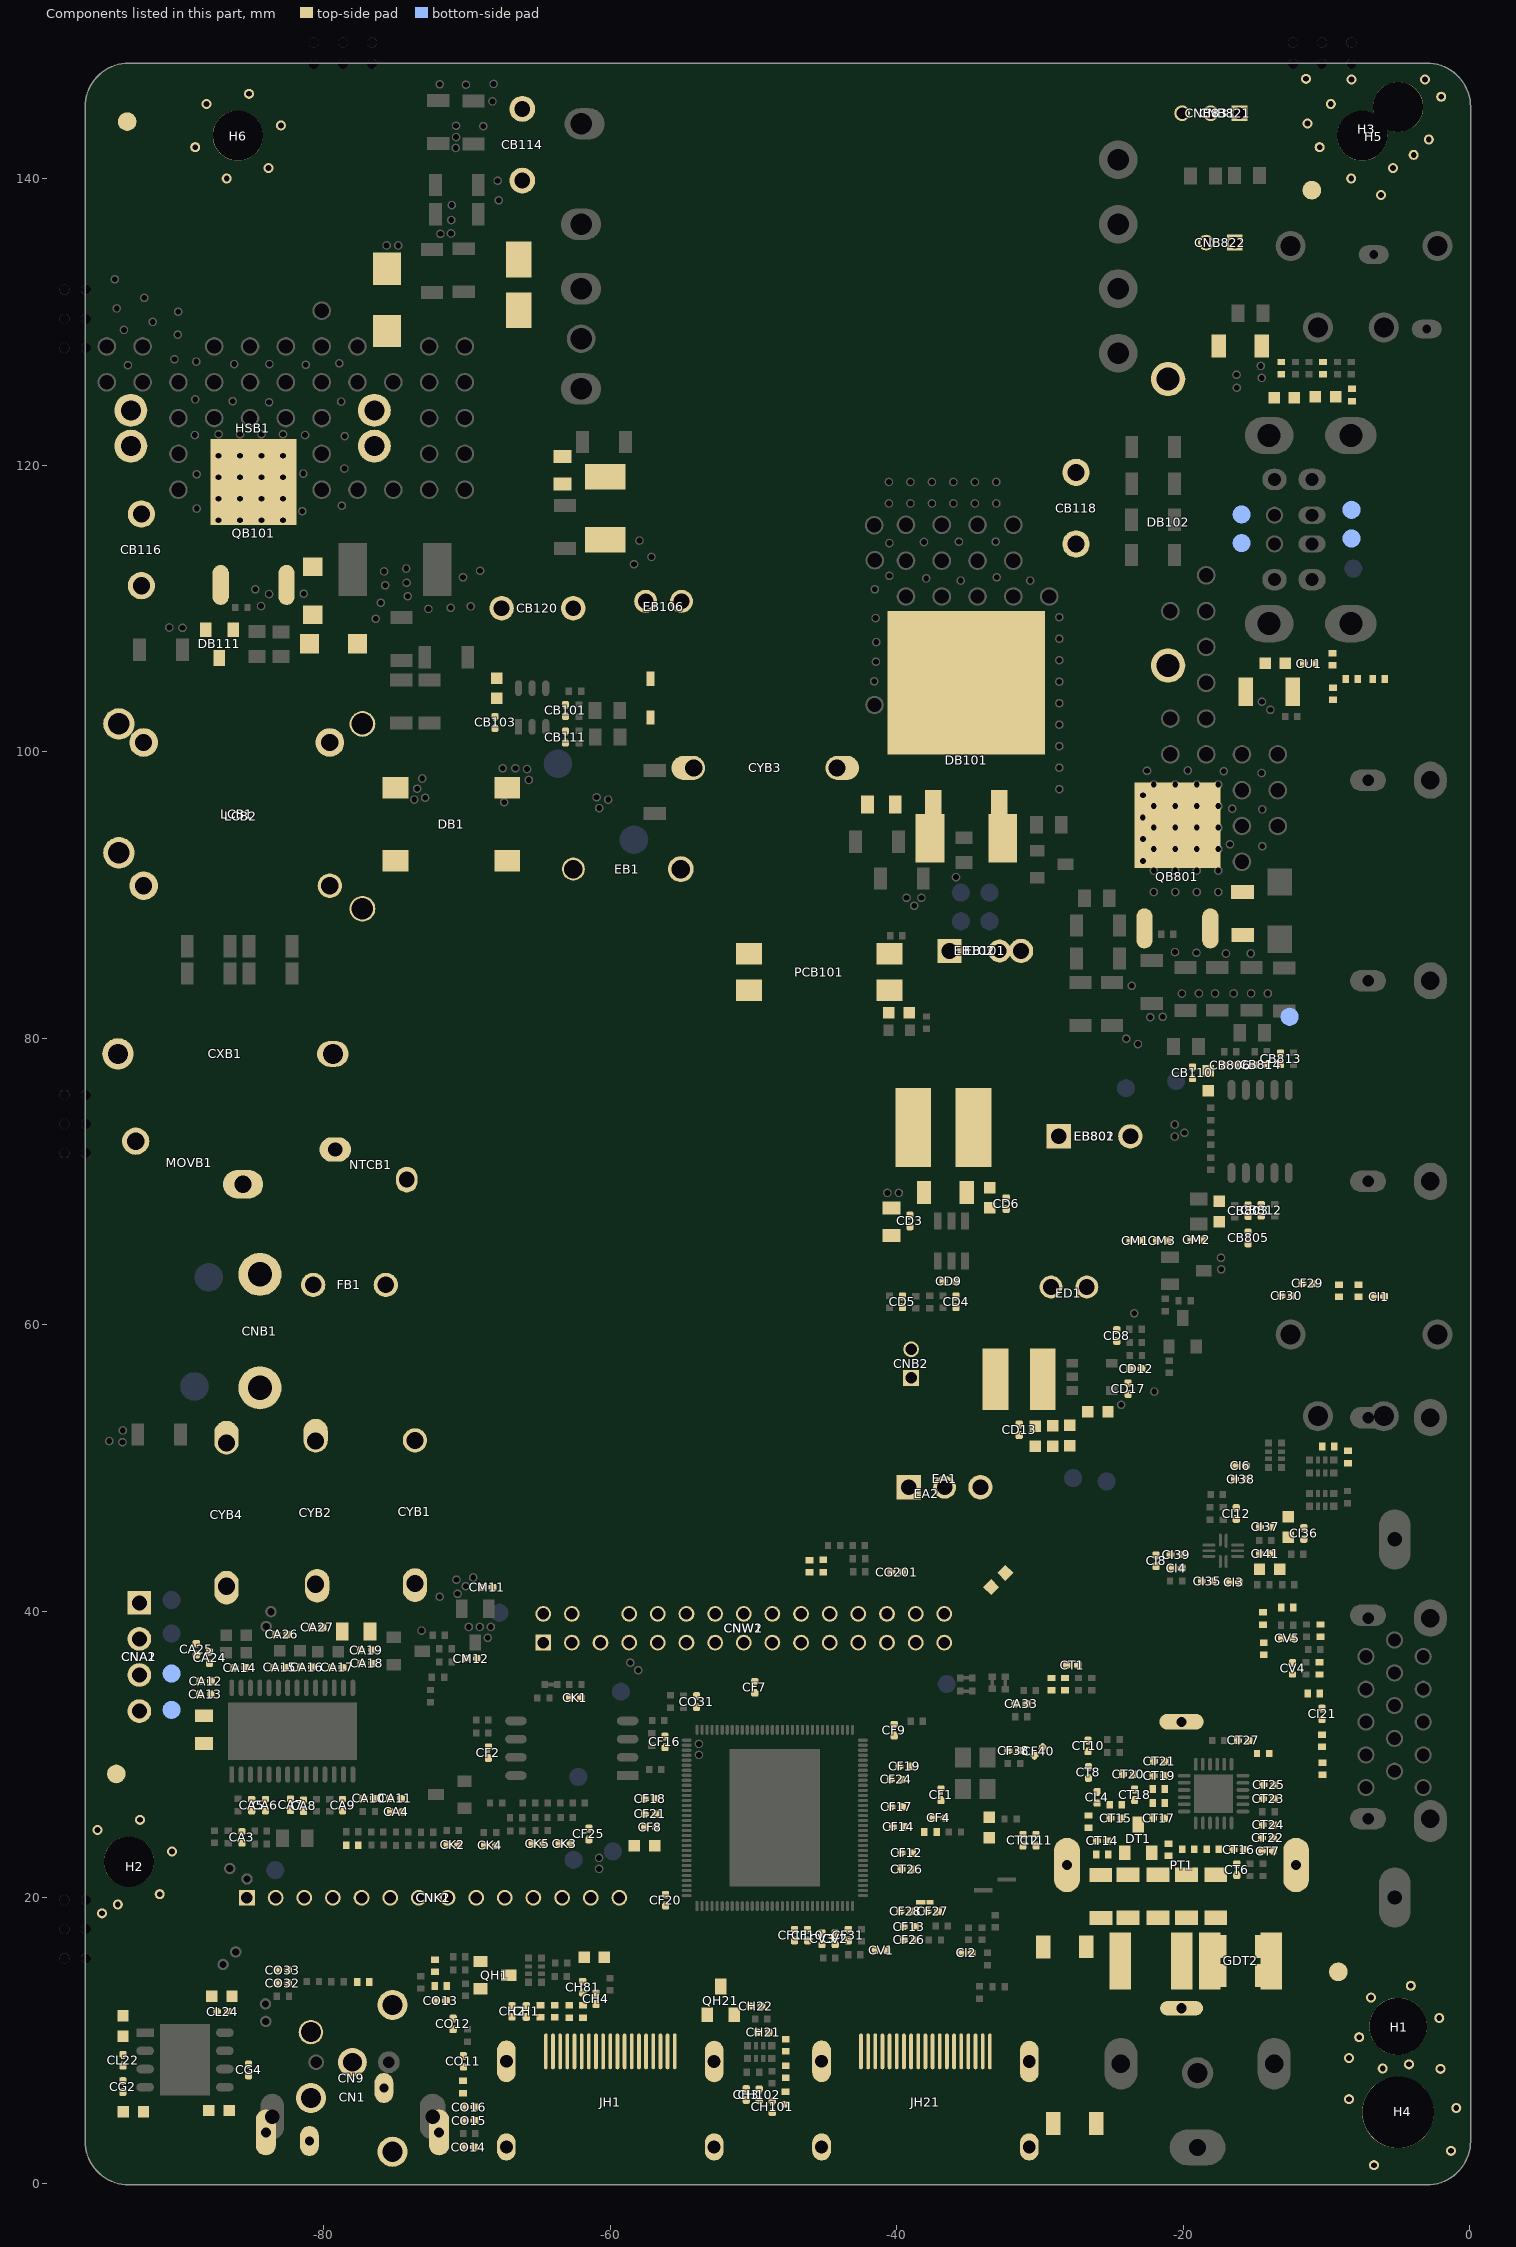
[diagram p0: the components of this part, seen from the top]
# Altium PCB MISC86372.PcbDoc (part 2 of 16)
Units mm, origin at the board's own origin, x right, y up, seen from the top; angles counter-clockwise.
Board outline 96.73 x 148.13 mm, 2 copper layers (TopLayer, BottomLayer), stack 1.571 mm thick; 578 components, 318 nets, 2702 pads, 836 vias.

## Components (designator, comment, footprint, x,y, rotation, side; value= is the part's Value field where it differs from the comment) (continued)
BB101 "Ferrite bead,BEAD,50ohm,3.0×4.0mm,9A,SMD,TP,BPH403025W4-470T,TAI-TECH" L(4*3*2.55)-S -66.396,132.585 r90 top
CA1 "10uF-0805-X5R-±20%-16V" C0805 -88.367,31.725 r90 top
CA2 "NC/10uF-0805-X5R-±20%-16V" C0805 -77.749,38.583 r180 top
CA3 "3300pF-0402-X7R-±10%-50V" C0402 -85.714,24.197 r90 top
CA4 "3300pF-0402-X7R-±10%-50V" C0402 -74.939,25.984 r180 top
CA5 "0.22uF-0402-X5R-±10%-16V" C0402 -85.033,26.448 r90 top
CA6 "0.22uF-0402-X5R-±10%-16V" C0402 -84.075,26.448 r90 top
CA7 "1uF-0402-X5R-±20%-16V" C0402 -82.324,26.468 r90 top
CA8 "1uF-0402-X5R-±20%-16V" C0402 -81.416,26.406 r90 top
CA9 "1uF-0402-X5R-±20%-16V" C0402 -78.689,26.448 r90 top
CA10 "0.22uF-0402-X5R-±10%-16V" C0402 -76.864,26.92 r180 top
CA11 "0.22uF-0402-X5R-±10%-16V" C0402 -74.994,26.921 r180 top
CA12 "NC/0.1uF-0402-X5R-±20%-16V" C0402 -88.243,35.105 r0 top
CA13 "1000pF-0402-X7R-±10%-50V" C0402 -88.268,34.188 r0 top
CA14 "0.22uF-0402-X5R-±10%-16V" C0402 -85.852,36.043 r0 top
CA15 "0.22uF-0402-X5R-±10%-16V" C0402 -83.077,36.069 r180 top
CA16 "0.22uF-0402-X5R-±10%-16V" C0402 -81.208,36.086 r0 top
CA17 "0.22uF-0402-X5R-±10%-16V" C0402 -79.063,36.068 r180 top
CA18 "NC/0.1uF-0402-X5R-±20%-16V" C0402 -76.995,36.347 r180 top
CA19 "1000pF-0402-X7R-±10%-50V" C0402 -77.025,37.272 r180 top
CA24 "2200pF-0402-X7R-±10%-50V" C0402 -87.979,36.751 r270 top
CA25 "2200pF-0402-X7R-±10%-50V" C0402 -88.9,37.338 r270 top
CA26 "2200pF-0402-X7R-±10%-50V" C0402 -82.927,38.372 r180 top
CA27 "2200pF-0402-X7R-±10%-50V" C0402 -80.463,38.869 r0 top
CA31 "10uF-0603-X5R-±20%-6.3V" C0603 -12.954,124.714 r180 top
CA32 "10uF-0603-X5R-±20%-6.3V" C0603 -10.062,124.765 r180 top
CA33 "Ceramic capacitor,CAP MC,6.3V,0.47uF,±10%,X5R,0402,SMD,TP" C0402 -31.323,33.528 r0 top
CAUTION "CAUTION" CAUTION -87.935,84.353 r90 bottom
CB101 "Ceramic capacitor,CAP MC,50V,100pF,±5%,NPO,0402,SMD,TP" C0402 -63.129,102.87 r270 top
CB102 "0.1uF-0603-X7R-±10%-50V" C0603 -67.92,104.419 r270 top
CB103 "Ceramic capacitor,CAP MC,50V,1000pF,±10%,X7R,0402,SMD,TP" C0402 -68.047,102.032 r90 top
CB109 "Ceramic capacitor,CAP MC,25V,0.22uF,±10%,X7R,0603,SMD,TP" C0603 -18.263,77.013 r270 top
CB110 "Ceramic capacitor,CAP MC,50V,100pF,±5%,NPO,0402,SMD,TP" C0402 -19.355,77.572 r270 top
CB111 "NC/Ceramic capacitor,CAP MC,50V,100pF,±5%,NPO,0402,SMD,TP" C0402 -63.129,101.016 r270 top
CB114 "Film capacitor,CAP PE,400V,4700pF,±5%,P,5.0mm,PC,DIP,TP,Fara" CAP8*2.5-V-5 -66.142,142.365 r90 top
CB116 "Ceramic capacitor,CAP CD,2KV,47pF,±5%,SL,IK,5.0mm,DIP,TP,Walsin" CAP7.5*5-V-5-1 -92.735,114.082 r270 top
CB117 "1000pF-0805-NPO-±10%-200V" C0805 -41.072,96.317 r180 top
CB118 "Ceramic capacitor,CAP CD,2KV,100pF,±5%,SL,IK,5.0mm,DIP,TP,Walsin" CAP8.5*5-V-5 -27.483,116.992 r270 top
CB119 "NC/1000pF-0805-NPO-±10%-200V" C0805 -63.348,119.634 r90 top
CB120 "NC/Ceramic capacitor,CAP CD,1KV,4700pF,±20%,Y5U,K,5.0mm,DIP,TP,Walsin" CAP10*4.5-V-5 -65.086,110.007 r0 top
CB129 "NC/Ceramic capacitor,CAP MC,1KV,1000pF,±5%,NPO,1206,SMD,TP" C1206 -15.85,88.697 r270 top
CB139 "NC/Ceramic capacitor,CAP MC,50V,0.022uF,±10%,X7R,0402,SMD,TP" C0603 -39.848,81.761 r180 top
CB801 "Ceramic capacitor,CAP MC,25V,1uF,±10%,X7R,0603,SMD,TP" C0603 -17.501,67.894 r270 top
CB803 "Ceramic capacitor,CAP MC,25V,0.1uF,±10%,X7R,0402,SMD,TP" C0402 -15.469,67.945 r270 top
CB805 "Ceramic capacitor,CAP MC,50V,0.01uF,±10%,X7R,0402,SMD,TP" C0402 -15.469,66.044 r270 top
CB806 "Ceramic capacitor,CAP MC,50V,1000pF,±10%,X7R,0402,SMD,TP" C0402 -16.713,78.105 r0 top
CB808 "NC/Ceramic capacitor,CAP MC,1KV,1000pF,±5%,NPO,1206,SMD,TP" C1206 -16.027,128.321 r180 top
CB812 "Ceramic capacitor,CAP MC,50V,220pF,±5%,NPO,0402,SMD,TP" C0402 -14.554,67.97 r90 top
CB813 "Ceramic capacitor,CAP MC,50V,100pF,±5%,NPO,0402,SMD,TP" C0402 -13.208,78.562 r270 top
CB814 "NC/100pF-0402-NPO-±5%-50V" C0402 -14.58,78.13 r180 top
CD1 "NC/10uF-1206-X5R-±10%-16V" C1206 -36.603,69.212 r180 top
CD2 "10uF-0805-X5R-±20%-16V" C0805 -40.361,67.168 r270 top
CD3 "NC/0.1uF-0402-X5R-±20%-16V" C0402 -39.079,67.231 r90 top
CD4 "0.1uF-0402-X5R-±20%-16V" C0402 -35.859,61.595 r90 top
CD5 "NC/56pF-0402-NPO-±5%-50V" C0402 -39.603,61.589 r270 top
CD6 "NC/0.1uF-0402-X5R-±20%-16V" C0402 -32.36,68.445 r90 top
CD7 "10uF-0603-X5R-±20%-6.3V" C0603 -33.503,68.845 r90 top
CD8 "0.1uF-0402-X5R-±20%-16V" C0402 -24.638,59.233 r90 top
CD9 "NC/0.1uF-0402-X5R-±20%-16V" C0402 -36.366,63.017 r0 top
CD10 "NC/10uF-0603-X5R-±20%-6.3V" C0603 -27.911,52.248 r270 top
CD12 "NC/NC/3300pF-0402-X7R-±10%-50V" C0402 -23.298,56.911 r0 top
CD13 "NC/0.1uF-0402-X5R-±20%-16V" C0402 -31.453,52.654 r270 top
CD14 "10uF-0603-X5R-±20%-6.3V" C0603 -29.115,52.222 r270 top
CD15 "10uF-0603-X5R-±20%-6.3V" C0603 -30.341,52.206 r270 top
CD16 "10uF-0603-X5R-±20%-6.3V" C0603 -25.96,53.904 r0 top
CD17 "NC/0.1uF-0402-X5R-±20%-16V" C0402 -23.849,55.525 r270 top
CD101 "NC/NC?" DIODE-S0402 -46.096,43.12 r90 top
CD102 "NC/NC?" DIODE-S0402 -45.131,43.145 r90 top
CF1 "Ceramic capacitor,CAP MC,50V,18pF,±5%,NPO,0402,SMD,TP" C0402 -36.906,27.178 r270 top
CF2 "0.1uF-0402-X5R-±20%-16V" C0402 -68.504,30.115 r270 top
CF3 "10uF-0603-X5R-±20%-6.3V" C0603 -57.615,23.628 r0 top
CF4 "Ceramic capacitor,CAP MC,50V,18pF,±5%,NPO,0402,SMD,TP" C0402 -37.058,25.552 r180 top
CF5 "10uF-0603-X5R-±20%-6.3V" C0603 -61.112,15.824 r180 top
CF7 "0.1uF-0402-X5R-±20%-16V" C0402 -49.911,34.671 r270 top
CF8 "0.1uF-0402-X5R-±20%-16V" C0402 -57.202,24.914 r0 top
CF9 "0.1uF-0402-X5R-±20%-16V" C0402 -40.174,31.689 r270 top
CF10 "0.1uF-0402-X5R-±20%-16V" C0402 -46.226,17.375 r90 top
CF11 "0.1uF-0402-X5R-±20%-16V" C0402 -47.14,17.375 r270 top
CF12 "0.1uF-0402-X5R-±20%-16V" C0402 -39.294,23.114 r180 top
CF13 "0.1uF-0402-X5R-±20%-16V" C0402 -39.115,17.975 r180 top
CF14 "0.1uF-0402-X5R-±20%-16V" C0402 -39.875,24.942 r180 top
CF15 "10uF-0603-X5R-±20%-6.3V" C0603 -32.918,42.164 r225 top
CF16 "0.1uF-0402-X5R-±20%-16V" C0402 -56.185,30.861 r270 top
CF17 "0.1uF-0402-X5R-±20%-16V" C0402 -40.005,26.34 r180 top
CF18 "0.1uF-0402-X5R-±20%-16V" C0402 -57.209,26.898 r180 top
CF19 "0.1uF-0402-X5R-±20%-16V" C0402 -39.446,29.159 r0 top
CF20 "0.1uF-0402-X5R-±20%-16V" C0402 -56.138,19.813 r90 top
CF21 "Ceramic capacitor,CAP MC,6.3V,0.47uF,±10%,X5R,0402,SMD,TP" C0402 -57.201,25.832 r180 top
CF24 "Ceramic capacitor,CAP MC,6.3V,2.2uF,±20%,X5R,0402,SMD,TP" C0402 -40.03,28.245 r0 top
CF25 "Ceramic capacitor,CAP MC,6.3V,0.47uF,±10%,X5R,0402,SMD,TP" C0402 -61.493,24.435 r90 top
CF26 "0.047uF-0402-X7R-±10%-16V" C0402 -39.116,17.043 r0 top
CF27 "NC/0.1uF-0402-X5R-±20%-16V" C0402 -37.484,19.043 r180 top
CF28 "1uF-0402-X5R-±20%-6.3V" C0402 -39.359,19.039 r0 top
CF29 "NC/1000pF-0402-X7R-±10%-50V" C0402 -11.303,62.865 r180 top
CF30 "NC/1000pF-0402-X7R-±10%-50V" C0402 -12.77,62.001 r0 top
CF31 "0.047uF-0402-X7R-±10%-16V" C0402 -43.383,17.374 r270 top
CF38 "NC/30pF-0402-NPO-±5%-50V" C0402 -31.833,30.251 r0 top
CF40 "Ceramic capacitor,CAP MC,50V,0.01uF,±10%,X7R,0402,SMD,TP" C0402 -30.099,30.201 r225 top
CG1 "10uF-0603-X5R-±20%-6.3V" C0603 -93.294,5.055 r180 top
CG2 "NC/Ceramic capacitor,CAP MC,6.3V,2.2uF,±20%,X5R,0402,SMD,TP" C0402 -94.027,6.802 r270 top
CG3 "NC/10uF-0603-X5R-±20%-6.3V" C0603 -87.323,5.13 r0 top
CG4 "1uF-0402-X5R-±20%-6.3V" C0402 -85.25,7.959 r270 top
CG201 "NC/0.1uF-0402-X5R-±20%-16V" C0402 -40.005,42.723 r0 top
CH1 "NC/0.1uF-0402-X5R-±20%-16V" C0402 -65.862,12.043 r90 top
CH2 "NC/0.1uF-0402-X5R-±20%-16V" C0402 -66.861,12.049 r90 top
CH3 "NC/Ceramic capacitor,CAP MC,50V,22pF,±5%,NPO,0402,SMD,TP" C0402 -50.506,6.244 r270 top
CH4 "NC/Ceramic capacitor,CAP MC,50V,22pF,±5%,NPO,0402,SMD,TP" C0402 -61.006,12.929 r270 top
CH21 "NC/0.1uF-0402-X5R-±20%-16V" C0402 -49.313,10.59 r0 top
CH22 "NC/0.1uF-0402-X5R-±20%-16V" C0402 -49.828,12.421 r180 top
CH81 "Ceramic capacitor,CAP MC,6.3V,0.47uF,±10%,X5R,0402,SMD,TP" C0402 -61.925,13.745 r90 top
CH101 "NC/10pF-0402-NPO-±5%-50V" C0402 -48.692,5.385 r270 top
CH102 "NC/10pF-0402-NPO-±5%-50V" C0402 -49.604,6.223 r90 top
CI1 "NC/10pF-0402-NPO-±5%-50V" C0402 -6.35,61.951 r180 top
CI2 "0.047uF-0402-X7R-±10%-16V" C0402 -35.154,16.129 r180 top
CI3 "NC/0.1uF-0402-X5R-±20%-16V" C0402 -16.472,41.993 r0 top
CI4 "NC/0.1uF-0402-X5R-±20%-16V" C0402 -20.496,42.996 r0 top
CI6 "0.1uF-0402-X5R-±20%-16V" C0402 -16.007,50.126 r0 top
CI8 "0.1uF-0402-X5R-±20%-16V" C0402 -21.895,43.51 r90 top
CI9 "NC/NC/10uF-0603-X5R-±20%-6.3V" C0603 -12.675,45.872 r270 top
CI12 "NC/Ceramic capacitor,CAP MC,6.3V,0.47uF,±10%,X5R,0402,SMD,TP" C0402 -16.298,46.805 r90 top
CI21 "NC/NC/10pF-0402-NPO-±5%-50V" C0402 -10.312,32.817 r270 top
CI35 "NC/1000pF-0402-X7R-±10%-50V" C0402 -18.335,42.088 r0 top
CI36 "NC/0.1uF-0402-X5R-±20%-16V" C0402 -11.582,45.415 r270 top
CI37 "NC/Ceramic capacitor,CAP MC,6.3V,0.47uF,±10%,X5R,0402,SMD,TP" C0402 -14.275,45.868 r0 top
CI38 "NC/Ceramic capacitor,CAP MC,6.3V,0.47uF,±10%,X5R,0402,SMD,TP" C0402 -16.002,49.2 r0 top
CI39 "NC/Ceramic capacitor,CAP MC,6.3V,0.47uF,±10%,X5R,0402,SMD,TP" C0402 -20.502,43.94 r180 top
CI40 "NC/10uF-0603-X5R-±20%-6.3V" C0603 -13.97,42.901 r180 top
CI41 "NC/0.1uF-0402-X5R-±20%-16V" C0402 -14.275,43.993 r180 top
CK1 "NC/22pF-0402-NPO-±5%-50V" C0402 -62.439,33.941 r0 top
CK2 "NC/0.1uF-0402-X5R-±20%-16V" C0402 -71,23.688 r0 top
CK3 "Ceramic capacitor,CAP MC,50V,0.01uF,±10%,X7R,0402,SMD,TP" C0402 -63.17,23.749 r180 top
CK4 "NC/0.1uF-0402-X5R-±20%-16V" C0402 -68.37,23.63 r180 top
CK5 "NC/0.1uF-0402-X5R-±20%-16V" C0402 -65.057,23.752 r0 top
CL3 "10uF-0603-X5R-±20%-6.3V" C0603 -33.55,24.889 r270 top
CL4 "NC/1uF-0402-X5R-±20%-6.3V" C0402 -26.01,26.988 r90 top
CL21 "10uF-0603-X5R-±20%-6.3V" C0603 -94.018,11.032 r90 top
CL22 "NC/Ceramic capacitor,CAP MC,6.3V,2.2uF,±20%,X5R,0402,SMD,TP" C0402 -94.018,8.64 r270 top
CL23 "NC/10uF-0603-X5R-±20%-6.3V" C0603 -87.114,13.106 r180 top
CL24 "1uF-0402-X5R-±20%-6.3V" C0402 -87.065,12.038 r0 top
CM1 "0.1uF-0402-X5R-±20%-16V" C0402 -23.306,65.863 r180 top
CM2 "NC/0.1uF-0402-X5R-±20%-16V" C0402 -19.053,65.913 r0 top
CM3 "NC/0.022uF-0402-X7R-±10%-16V" C0402 -21.452,65.862 r180 top
CM11 "NC/0.1uF-0402-X5R-±20%-16V" C0402 -68.595,41.652 r180 top
CM12 "0.022uF-0402-X7R-±10%-16V" C0402 -69.693,36.68 r180 top
CN1 "NC/RCA jack,RCA Jack,AV1,H,Yellow,CH5.5,Seal,DIP,AV38A-01S-5030,QS" AV1-H-4 -78,0.45 r0 top locked
CN9 "NC/Earphone jack,Earphone Jack,H,Φ3.5,CH7.0,Black,switch,Seal,DIP,PJ-373A,JSL" PHONE-HD-42#2 -78,0 r0 top locked
CNA1 "Connector socket,connect jack,4Pin,D2.5,D,Nature,L=2.8mm,DIP,W2411-04SVA-ENSY,XYDT" SIP4/2.54D-1 -92.877,36.793 r270 top locked
CNA2 "NC/4PIN-2.54-D-H-G-latched-B" SIP4/2.5D-2 -92.877,36.793 r270 top
CNB1 "Connector socket,connect jack,2Pin,D7.92,L,SNAP,Fool-proofing,Nature,L=2.8mm,DIP,W7913-02RVA-S39SY,XYDT" CON2-H7.92 -84.455,59.54 r0 top
CNB2 "Connector socket,connect jack,2Pin,D2.0,D,Beige,L=2.8mm,DIP,W2011-02SVA-SN8-ENSY,XYDT" SIP2/2.0D-1 -39,57.275 r90 top
CNB821 "Connector socket,connect jack,2Pin,D2.0,D,Beige,L=2.8mm,DIP,W2011-02SVA-SN8-ENSY,XYDT" SIP2/2.0D-CP -17.081,144.562 r180 top
CNB822 "NC/Connector socket,connect jack,2Pin,D2.0,D,L=2.8mm,DIP,AMA" SIP2/2.0D-CP -17.408,135.534 r180 top
CNB831 "NC/Connector socket,connect jack,3Pin,D2.0,D,L=2.8mm,DIP,AMA" SIP3/2.0D-CP -18.081,144.562 r180 top
CNK1 "NC/Connector socket,connect jack,14Pin,D2.0,D,SNAP,Nature,L=2.8mm,DIP,AMA" SIP14/2.0D-5 -72.365,19.99 r0 top locked
CNK2 "Connector socket,connect jack,14Pin,D2.0,D,Fool-proofing,Nature,L=2.8,DIP,W2011-14SVA-SN9-ENSY,XYDT" SIP14/2.0D-1 -72.365,19.99 r0 top locked
CNW1 "NC/NC/Connector socket,connect jack,2×15Pin/without pin6,D2.0,D,SNAP,Fool-proofing,Nature,L=2.6mm,DIP,CJ" SIP2*15/2.0D-11 -50.682,38.796 r180 top locked
CNW2 "Gold pin,pin connector,2×15Pin/without pin6,D,D2.0mm,L=2.6mm,DIP,H2030-30SVB-V06-J8SY,XYDT" SIP2*15/2.0D-2 -50.681,38.796 r180 top locked
CO11 "NC/1000pF-0402-X7R-±10%-50V" C0402 -70.256,8.56 r90 top
CO12 "NC/Ceramic capacitor,CAP MC,6.3V,0.47uF,±10%,X5R,0402,SMD,TP" C0402 -70.968,11.176 r270 top
CO13 "NC/1000pF-0402-X7R-±10%-50V" C0402 -71.831,12.802 r180 top
CO14 "NC/1000pF-0402-X7R-±10%-50V" C0402 -69.887,2.577 r0 top
CO15 "NC/Ceramic capacitor,CAP MC,6.3V,0.47uF,±10%,X5R,0402,SMD,TP" C0402 -69.85,4.431 r0 top
CO16 "NC/1000pF-0402-X7R-±10%-50V" C0402 -69.85,5.371 r180 top
CO31 "NC/NC/33pF-0402-NPO-±5%-50V" C0402 -53.975,33.68 r90 top
CO32 "0.1uF-0402-X5R-±20%-16V" C0402 -82.855,14.021 r180 top
CO33 "330pF-0402-NPO-±5%-50V" C0402 -82.855,14.935 r0 top
COLD "COLD" COLD -38.608,118.466 r0 top
"Conformal Coating" "NC/Conformal coating,25kg/Can,Peters" "Conformal Coating" -57.226,70.079 r90 top
CQC "CQC" CQC -37.49,72.923 r270 top
CT1 "NC/0.1uF-0402-X5R-±20%-16V" C0402 -27.737,36.22 r180 top
CT6 "Ceramic capacitor,CAP MC,50V,22pF,±5%,NPO,0402,SMD,TP" C0402 -16.259,21.95 r90 top
CT7 "Ceramic capacitor,CAP MC,50V,22pF,±5%,NPO,0402,SMD,TP" C0402 -14.117,23.239 r180 top
CT8 "NC/30pF-0402-NPO-±5%-50V" C0402 -26.619,28.727 r90 top
CT10 "NC/30pF-0402-NPO-±5%-50V" C0402 -26.645,30.582 r90 top
CT11 "0.1uF-0402-X5R-±20%-16V" C0402 -30.277,24.003 r90 top
CT12 "0.1uF-0402-X5R-±20%-16V" C0402 -31.191,24.003 r90 top
CT13 "Ceramic capacitor,CAP MC,1KV,470pF,±5%,NPO,1206,SMD,TP" C1206 -23.851,20.091 r90 top
CT14 "NC/220pF-0402-NPO-±5%-50V" C0402 -25.654,23.952 r180 top
CT15 "0ohm-0402-±5%-1/16W" C0402 -24.707,25.535 r0 top
CT16 "0.047uF-0402-X7R-±10%-16V" C0402 -16.129,23.343 r0 top
CT17 "0.1uF-0402-X5R-±20%-16V" C0402 -21.717,25.532 r0 top
CT18 "NC/1000pF-0402-X7R-±10%-50V" C0402 -23.393,27.178 r270 top
CT19 "0.022uF-0402-X7R-±10%-16V" C0402 -21.692,28.504 r0 top
CT20 "0.022uF-0402-X7R-±10%-16V" C0402 -23.829,28.6 r180 top
CT21 "0.1uF-0402-X5R-±20%-16V" C0402 -21.666,29.515 r0 top
CT22 "0.1uF-0402-X5R-±20%-16V" C0402 -14.117,24.154 r0 top
CT23 "330pF-0402-NPO-±5%-50V" C0402 -14.049,26.903 r180 top
CT24 "6800pF-0402-X7R-±10%-50V" C0402 -14.072,25.07 r180 top
CT25 "0.1uF-0402-X5R-±20%-16V" C0402 -14.021,27.864 r0 top
CT26 "0.022uF-0402-X7R-±10%-16V" C0402 -39.294,21.971 r180 top
CT27 "0.1uF-0402-X5R-±20%-16V" C0402 -15.799,30.963 r180 top
CT41 "Thick-film resistor,RES,1/4W,0ohm,±5%,1206,SMD" C1206 -25.756,20.066 r270 top
CT42 "Thick-film resistor,RES,1/4W,0ohm,±5%,1206,SMD" C1206 -21.768,20.091 r270 top
CT43 "Thick-film resistor,RES,1/4W,0ohm,±5%,1206,SMD" C1206 -19.761,20.091 r270 top
CT44 "Thick-film resistor,RES,1/4W,0ohm,±5%,1206,SMD" C1206 -17.729,20.091 r270 top
CT45 "Thick-film resistor,RES,1/4W,0ohm,±5%,1206,SMD" C1206 -15.977,16.586 r180 top
CT46 "Thick-film resistor,RES,1/4W,0ohm,±5%,1206,SMD" C1206 -15.977,14.554 r180 top
CT47 "NC/Ceramic capacitor,CAP MC,1KV,4700pF,±10%,X7R,1206,SMD,TP" C1206 -28.27,16.56 r0 top
CT48 "NC/Ceramic capacitor,CAP MC,1KV,4700pF,±10%,X7R,1206,SMD,TP" C1206 -27.584,4.211 r0 top
CU1 "1uF-0402-X5R-±20%-6.3V" C0402 -11.198,106.147 r0 top
CU2 "NC/10uF-0603-X5R-±20%-6.3V" C0603 -13.578,106.153 r180 top
CV1 "0.047uF-0402-X7R-±10%-16V" C0402 -41.097,16.307 r180 top
CV2 "0.047uF-0402-X7R-±10%-16V" C0402 -44.298,17.12 r90 top
CV3 "0.047uF-0402-X7R-±10%-16V" C0402 -45.215,17.12 r90 top
CV4 "NC/30pF-0402-NPO-±5%-50V" C0402 -12.37,35.992 r90 top
CV5 "NC/30pF-0402-NPO-±5%-50V" C0402 -12.739,38.093 r180 top
CXB1 "X capacitor,CAP X2,MP,280VAC,0.33uF,±10%,S,15mm,PC,DIP,JH" CAP18*8.5-V-15 -86.868,78.892 r180 top
CYB1 "Y capacitor,CAP Y1,CD,470pF,400VAC,±20%,KS,10mm,Y5U,DIP,Walsin" CAP13*5-V-10-1#1 -73.635,46.914 r270 top
CYB2 "Y capacitor,CAP Y1,CD,470pF,400VAC,±20%,KS,10mm,Y5U,DIP,Walsin" CAP13*5-V-10-1#2 -80.569,46.867 r270 top
CYB3 "Y capacitor,CAP Y1,CD,470pF,400VAC,±20%,KS,10mm,Y5U,DIP,Walsin" CAP13*5-V-10-1#3 -49.178,98.857 r0 top
CYB4 "NC/Y capacitor,CAP Y1,CD,220pF,400VAC,±10%,K,10mm,Y5P,DIP,TP,Walsin" CAP13*5-V-10-1#4 -86.792,46.732 r270 top
DA31 "NC/NC?" DIODE-S0402 -10.251,126.771 r90 top
DA32 "NC/NC?" DIODE-S0402 -13.157,126.771 r90 top
DA33 "NC/NC?" DIODE-S0402 -8.23,124.894 r90 top
DB1 "Bridge rectifier,DIO BRD,3A,800V,YBS,SMD,YBS3010A,YJ" B/YBS3010A -71.095,94.92 r270 top
DB101 "Schottky diode,DIO SBD D1,10A,150V,TO-252,SMD,MBR10150GCT,PINGWEI" D2PAK3 -35.242,101.452 r270 top
DB102 "Rectifier diode,DIO FRD S,4A,600V,DO-201AD,DIP,MUR460,GULF" D3-H-20 -21.057,116.009 r270 top
DB104 "Rectifier diode,DIO SI S,1A,1000V,SMAF,SMD,M7F,YJ" DIODE-S-2 -60.35,116.992 r270 top
DB106 "Rectifier diode,DIO FRD S,2A,800V,DO-214AC,SMD,GR2KA,GOOD-ARK" DIODE-SMA-2 -75.59,131.536 r90 top
DB107 "Switching diode,DIO SW S,200mA,250V,SOD-323,SMD,BAV21WS,BLUE ROCKET" DIODE-S-12 -57.201,103.734 r270 top
DB109 "Rectifier diode,DIO FRD S,1.2A,800V,SOD-123FL,SMD,F1K,YJ" DIODE-S-14 -80.772,111.227 r90 top
DB110 "Rectifier diode,DIO FRD S,1.2A,800V,SOD-123FL,SMD,F1K,YJ" DIODE-S-14 -79.324,107.518 r180 top
DB111 "Switching diode,DIO SW D1,215mA,85V,SOT-23,SMD,KAV70,KEXIN" SO-23 -87.287,107.493 r0 top
DBS0 "DOLBY" DOLBY-SILK -23.546,28.6 r180 bottom
DH1 "Ceramic capacitor,CAP MC,50V,22pF,±5%,NPO,0402,SMD,TP" DIODE-S0402 -61.906,12.04 r270 top
DH2 "NC/SFI0402-240E-2R5PP-LF" DIODE-S0402 -63.881,12.065 r270 top
DH3 "NC/SFI0402-240E-2R5PP-LF" DIODE-S0402 -64.861,12.065 r270 top
DH21 "Ceramic capacitor,CAP MC,50V,22pF,±5%,NPO,0402,SMD,TP" DIODE-S0402 -47.777,6.002 r90 top
DH22 "NC/SFI0402-240E-2R5PP-LF" DIODE-S0402 -47.752,7.828 r90 top
DH23 "NC/SFI0402-240E-2R5PP-LF" DIODE-S0402 -47.752,9.677 r270 top
DH81 "NC/SFI0402-240E-2R5PP-LF" DIODE-S0402 -62.865,12.04 r270 top
DI1 "NC/AVLC18S02003" DIODE-S0402 -14.378,37.373 r270 top
DI2 "NC/AVLC18S02003" DIODE-S0402 -9.119,62.357 r90 top
DI3 "NC/AVLC18S02003" DIODE-S0402 -7.772,62.357 r90 top
DI6 "NC/NC/AVLC18S02003" DIODE-S0402 -71.831,13.818 r180 top
DI8 "NC/NC/SFI0402-240E-2R5PP-LF" DIODE-S0402 -70.275,6.768 r270 top
DI9 "NC/NC/SFI0402-240E-2R5PP-LF" DIODE-S0402 -77.241,14.101 r180 top
DK1 "NC/AVLC18S02003" DIODE-S0402 -78.01,23.648 r0 top
DK2 "NC/AVLC18S02003" DIODE-S0402 -28.245,34.9 r270 top
DK3 "NC/AVLC18S02003" DIODE-S0402 -29.21,34.9 r270 top
DM0 "DM0" TP -15.925,114.556 r180 bottom
DM1 "DM0" TP -8.251,114.876 r180 bottom
DO1 "NC/AVLC18S02003" DIODE-S0402 -72.238,15.24 r270 top
DP0 "DM0" TP -15.925,116.556 r180 bottom
DP1 "DM0" TP -8.251,116.876 r180 bottom
DT1 "KAV99" SO-23 -23.139,24.13 r180 top
DU1 "NC/TVS diode,DIO ESD,0.1pF,25V,0402,SMD,GESD1005H150CR10GPT,Sunlord" DIODE-S0402 -6.35,105.054 r180 top
DU2 "NC/TVS diode,DIO ESD,0.1pF,25V,0402,SMD,GESD1005H150CR10GPT,Sunlord" DIODE-S0402 -8.23,105.054 r0 top
DU3 "NC/TVS diode,DIO ESD,0.1pF,25V,0402,SMD,GESD1005H150CR10GPT,Sunlord" DIODE-S0402 -9.55,104.038 r90 top
DU4 "NC/TVS diode,DIO ESD,0.1pF,25V,0402,SMD,GESD1005H150CR10GPT,Sunlord" DIODE-S0402 -9.576,106.451 r270 top
DV1 "NC/AVLC18S02003" DIODE-S0402 -12.733,40.234 r0 top
DV2 "NC/AVLC18S02003" DIODE-S0402 -14.427,39.478 r270 top
DV3 "NC/AVLC18S02003" DIODE-S0402 -10.897,34.239 r0 top
DV4 "NC/AVLC18S02003" DIODE-S0402 -10.287,28.981 r90 top
DV5 "NC/AVLC18S02003" DIODE-S0402 -10.312,30.937 r90 top
DV6 "NC/AVLC18S02003" DIODE-S0402 -10.49,35.992 r90 top
DV7 "NC/AVLC18S02003" DIODE-S0402 -10.431,38.633 r90 top
DV8 "NC/AVLC18S02003" DIODE-S0402 -9.881,51.486 r180 top
DV9 "NC/AVLC18S02003" DIODE-S0402 -8.509,50.749 r270 top
EA1 "Aluminium electrolytic capacitor,CAP AL,16V,470uF,±20%,KM,P,5.0mm,10×12.5,DIP,TP,Samxon" EC(10*12)-V-5 -36.658,48.643 r0 top locked
EA2 "NC/Aluminium electrolytic capacitor,CAP AL,16V,220uF,±20%,LD,KF,P,2.5mm,6.3×11,DIP,TP,CapXon" EC(6.3*11)-V-2.5#1 -37.908,48.643 r0 top locked
EB1 "Aluminium electrolytic capacitor,CAP AL,400V,100uF,±20%,KM,BK,7.5mm,16×31.5,DIP,CapXon" EC(18*31.5)-H-7.5 -58.826,91.796 r0 top
EB101 "Aluminium electrolytic capacitor,CAP AL,25V,470uF,±20%,LD,PKLH,P,5.0mm,10×12.5,DIP,TP,Koshin" EC(10*12.5)-V-5#1 -33.823,86.081 r0 top
EB102 "NC/270uF-16V-±20%-8×11.5-105℃-PS-short leg-F=3.5(Capxon)" EC(8*11)-V-3.5 -34.573,86.081 r0 top
EB106 "10uF-50V-±20%-5×11-105℃-GH-tape-reel-F=2.5(CapXon)" EC(5*11)-V-2.5 -56.281,110.49 r0 top
EB801 "Aluminium electrolytic capacitor,CAP AL,100V,47uF,±20%,LD,PKLW,P,5.0mm,10×12.5,DIP,TP,Koshin" EC(10*12.5)-V-5#2 -26.187,73.139 r0 top
EB802 "NC/Aluminium electrolytic capacitor,CAP AL,160V,39uF,±20%,LD,ZD,P,5.0mm,12.5×12,DIP,TP,HEC" EC(13*13)-V-5 -26.187,73.139 r0 top
ED1 "Aluminium electrolytic capacitor,CAP AL,10V,470uF,±20%,PKZH,P,2.5mm,6.3×11,DIP,TP,Koshin" EC(6.3*11)-V-2.5#2 -27.978,62.619 r0 top locked
EVA1 "NC/7×7×3mm-C-4305 fire-retardant foam-black" EVA(7*7*3) -84.861,124.104 r180 bottom
EVA2 "NC/7×7×3mm-C-4305 fire-retardant foam-black" EVA(7*7*3) -35.331,114.5 r180 bottom
EVA3 "NC/7×7×3mm-C-4305 fire-retardant foam-black" EVA(7*7*3) -70.587,82.372 r180 bottom
EVA4 "NC/7×7×3mm-C-4305 fire-retardant foam-black" EVA(7*7*3) -48.285,19.406 r180 bottom
EVA5 "NC/7×7×3mm-C-4305 fire-retardant foam-black" EVA(7*7*3) -90.238,7.391 r180 bottom
EVA6 "NC/7×7×3mm-C-4305 fire-retardant foam-black" EVA(7*7*3) -15.824,38.252 r180 bottom
FB1 "Slow-blow fuse,FUSE T,P,3.15A,250VAC,8.5×4.0×8mm,DIP,TP,Walter" "FUSE8.5*4-V-5(T3.15AL 250V~)" -78.207,62.763 r180 top
FU1 "NC/NSMD110(1206-1.1A)" FUSE1.1A-S -13.994,104.165 r180 top
GD1 "NC/7.00×8.35mm-nylon-white-WQM" Fixed -47.5,92 r180 bottom locked
GD2 "NC/7.00×8.35mm-nylon-white-WQM" Fixed -76.5,143 r0 top locked
GD3 "NC/7.00×8.35mm-nylon-white-WQM" Fixed -68,48 r0 top locked
GDT1 "NC/Gas discharge tube,GDT,700V,2000A,TP,4.5*3.2mm,SMD,4532-091-LF,Brightking" SMD4532-1 -22.25,15.57 r0 top
GDT2 "NC/Gas discharge tube,GDT,700V,2000A,TP,4.5*3.2mm,SMD,4532-091-LF,Brightking" SMD4532-1-C1206 -16.002,15.57 r270 top
GL1 "Silicone,0.5g,general,60,white,SLD-8854W,XY" "Silica gel-15" -69.24,62.992 r0 top
H1 "Location hole" ASSE4.0C-3 -5,11 r0 top locked
H2 "Location hole" ASSE3.5C-3#1 -93.6,22.5 r0 top locked
H3 "Location hole" ASSE3.5C-3#2 -7.5,143 r0 top locked
H4 "Location hole" ASSE5.0C-3 -5,5 r0 top locked
H5 "Location hole" ASSE3.5C-3#3 -5,145 r0 top locked
H6 "Location hole" ASSE3.5C-3#4 -86,143 r0 top locked
"High Voltage" "High Voltage" "High Voltage" -64.904,90.423 r0 top
HOT "HOT" HOT -66.37,122.453 r90 top
HS1 "NC/Heatsink,6-series aluminium alloy,14.0×14.0×6.0mm,natural,XXWJ" HS(14*14*6) -48.513,25.556 r0 top locked
HSB1 "NC/Heatsink,17.5×14.5×0.5mm,red copper sheet,matte tin plated,natural,four pins,WT" HS149-YZ -84.972,122.575 r180 top
JH1 "HDMI jack,HDMI Jack,H,SMD,161031041(hull-SPCC ),VAST" HDMI-HS-1#1 -60,-2 r0 top locked
JH21 "HDMI jack,HDMI Jack,H,SMD,161031041(hull-SPCC ),VAST" HDMI-HS-1#2 -38,-2 r0 top locked
L3 "0ohm-0402-±5%-1/16W" L0402 -37.643,24.563 r180 top
L6 "0ohm-0402-±5%-1/16W" R0402 -14.427,30.041 r180 top
LCB1 "NC/Common-mode choke,Common Choke,UU10.5,18mH MIN,0.35×1P,80Ts,H14.5MAX,SYUU10.5-L002,DIP,EDL" L/UU10.5/10*13-2 -86.078,95.635 r270 top
LCB2 "Common-mode choke,Common Choke,UC15Z,10.5mH,0.13×1.0mm,48Ts,H14.0MAX,SYUC15-L10.5mA,DIP,DX" L/LC4/20.5*16-H-17*9(12.9) -85.801,95.479 r0 top
LD1 "Power inductor,Power Inductor,4.7uH,±20%,2.8A,0.32×1P,DR5.8×4.5,SMD,CKO54-4.7uH/M,CK" L(5.8*4.5)-S -36.738,73.746 r180 top
LD2 "Power inductor,Power Inductor,2.2uH,±20%,2A,0.28×1P,DR4.5×3.2,SMD,PIO43-2R2MTP02,FH" L(4.5*3.5)-S -31.453,56.185 r0 top
LF6 "NC/?" GND#1 -37.998,19.66 r180 top
LOUT+ "DM0" TP -90.627,33.096 r180 bottom
LOUT- "DM0" TP -90.627,35.636 r180 bottom
LT2 "NC/SDCL1005CR27JTDF(Sunlord)" L0402 -25.654,23.012 r180 top
LT3 "NC/SDCL1005CR18JTDF(180nH-0402±5%-C)" L0402 -26.619,25.298 r90 top
LT4 "GZ1005U102CTF(1000ohm-300mA)" L0402 -21.031,23.343 r270 top
LT5 "GZ1005U102CTF(1000ohm-300mA)" L0402 -19.66,23.368 r180 top
LT6 "SDCL1005CR18JTDF(180nH-0402±5%-C)" L0402 -17.932,23.368 r180 top
LT8 "Multilayer inductor,,HF Inductor,39nH,±5%,0402,SMD,SDCL1005C39NJTDF,Sunlord" L0402 -21.717,26.599 r0 top
LT9 "Multilayer inductor,HF Inductor,270nH,±5%,0402,SMD,SDCL1005CR27JTDF,Sunlord" L0402 -21.717,27.564 r180 top
LT10 "NC/SDCL1005CR18JTDF(180nH-0402±5%-C)" L0402 -24.707,26.474 r180 top
M1 "MARK" MARK -94.488,28.626 r0 top
M2 "MARK" MARK -11.024,139.192 r0 top
M3 "MARK" MARK -93.726,143.98 r0 top
M4 "MARK" MARK -9.173,14.811 r0 top
Manufacture_Info "Manufacture_Info" Manufacture_Info -31.626,103.746 r180 top
ML1 "NC/Latest Mylar sheet" Mylar -57.234,70.174 r90 top
MOVB1 "NC/Varistor,VARISTOR,128J,680V,4000A,S,7.5mm,10mm,DIP,Thinking" VR(13*5)-V-7.5 -89.383,71.298 r0 top
NTCB1 "NTC thermistor,RES NTC,2.4W,5A,2.5ohm,±20%,S,5.0mm,10mm,DIP,JOYIN" NTC(10*5)-V5 -76.708,71.171 r180 top
PCB101 "LTV-817S-TA-B(Lite-On)" OC4-S-1 -45.415,84.607 r90 top
PT1 "Shield can,tinplate,natural,20.3×16.3×6mm,with sealed opening,LHD" SHIELD(16*20*6) -20.117,12.268 r0 top locked
PWM_REF "" TP_BL -12.573,81.483 r270 bottom
QB101 "Field-effect transistor,NMOS,7A,650V,0.55ohm@ID=3.5A@VGS=10V,TO-252,LSG65R650HT,LONTEN" TO-252-GDS -84.901,118.833 r0 top
QB801 "Field-effect transistor,MOSFET,20A,150V,71mohm@ID=10A@VGS=10V,TO-252-2L,NCEP1520K,NCEPOWER" TO-252-GDS -20.408,94.855 r0 top
QH1 "General transistor,Dynatron,NPN,0.2A,40V,30-300,SOT-23,MMBT3904(f≥350MHz),BLUE ROCKET" SOT-23 -68.047,14.58 r90 top
QH21 "General transistor,Dynatron,NPN,0.2A,40V,30-300,SOT-23,MMBT3904(f≥350MHz),BLUE ROCKET" SOT-23 -52.286,12.827 r180 top